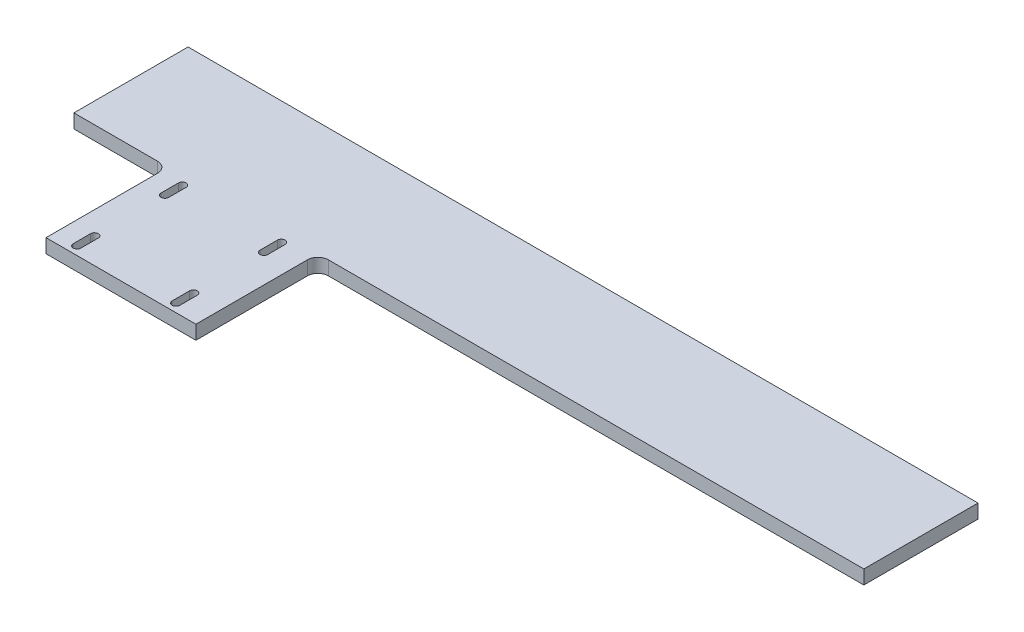
SolidWorks part; units mm, degrees
ref_plane "前视基准面" through (0, 0, 0) normal (0, 0, 1) x (1, 0, 0)
ref_plane "上视基准面" through (0, 0, 0) normal (0, 1, 0) x (1, 0, 0)
ref_plane "右视基准面" through (0, 0, 0) normal (1, 0, 0) x (0, 0, -1)
sketch "草图1" plane through (0, 0, 0) normal (0, 1, 0) x (1, 0, 0)
  line L1 (-1133, -163.75) -> (1133, -163.75)
  line L2 (-1133, -163.75) -> (-1133, 163.75)
  line L3 (-1133, 163.75) -> (1133, 163.75)
  line L4 (1133, -163.75) -> (1133, 163.75)
  line L5 (-1133, -163.75) -> (1133, 163.75) construction
  line L6 (-1133, 163.75) -> (1133, -163.75) construction
  point P0 (0, 0)
  dimension "D1" = 2266
  dimension "D2" = 327.5
extrude "凸台-拉伸1" add sketch "草图1" along normal blind 40
sketch "草图2" plane through (0, 40, 0) normal (0, 1, 0) x (1, 0, 0)
  line L0 (-1133, -163.75) -> (1133, -163.75) construction
  line L1 (-433, -163.75) -> (-863, -163.75)
  line L2 (-433, -163.75) -> (-433, -513.75)
  line L3 (-433, -513.75) -> (-863, -513.75)
  line L4 (-863, -163.75) -> (-863, -513.75)
  line L5 (-1133, 163.75) -> (-1133, -163.75) construction
  dimension "D1" = 700
  dimension "D2" = 430
  dimension "D3" = 350
extrude "凸台-拉伸2" add sketch "草图2" against normal blind 40
sketch "草图3" plane through (0, 40, 0) normal (0, 1, 0) x (1, 0, 0)
  line L0 (-514, -187.75) -> (-514, -237.75) construction
  line L1 (-503, -187.75) -> (-503, -237.75)
  line L2 (-525, -187.75) -> (-525, -237.75)
  line L3 (-433, -513.75) -> (-433, -163.75) construction
  line L4 (-514, -439.75) -> (-514, -489.75) construction
  line L7 (-863, -513.75) -> (-433, -513.75) construction
  line L8 (-798, -187.75) -> (-798, -237.75) construction
  line L9 (-787, -187.75) -> (-787, -237.75)
  line L10 (-809, -187.75) -> (-809, -237.75)
  line L11 (-798, -439.75) -> (-798, -489.75) construction
  line L12 (-787, -439.75) -> (-787, -489.75)
  line L13 (-809, -439.75) -> (-809, -489.75)
  line L14 (-503, -439.75) -> (-503, -489.75)
  line L15 (-525, -439.75) -> (-525, -489.75)
  line L16 (-1133, 163.75) -> (-1133, -163.75) construction
  line L17 (1133, 163.75) -> (-1133, 163.75) construction
  arc A0 (-503, -187.75) -> (-525, -187.75) centre (-514, -187.75) ccw
  arc A1 (-525, -237.75) -> (-503, -237.75) centre (-514, -237.75) ccw
  circle A2 centre (-514, -187.75) radius 11 construction
  arc A7 (-787, -187.75) -> (-809, -187.75) centre (-798, -187.75) ccw
  arc A8 (-809, -237.75) -> (-787, -237.75) centre (-798, -237.75) ccw
  circle A9 centre (-798, -187.75) radius 11 construction
  arc A10 (-787, -439.75) -> (-809, -439.75) centre (-798, -439.75) ccw
  arc A11 (-809, -489.75) -> (-787, -489.75) centre (-798, -489.75) ccw
  circle A12 centre (-798, -439.75) radius 11 construction
  arc A13 (-503, -439.75) -> (-525, -439.75) centre (-514, -439.75) ccw
  arc A14 (-525, -489.75) -> (-503, -489.75) centre (-514, -489.75) ccw
  circle A15 centre (-514, -439.75) radius 11 construction
  point P2 (-514, -212.75)
  point P12 (-514, -464.75)
  point P23 (-798, -212.75)
  point P32 (-798, -464.75)
  dimension "D6" = 11
  dimension "D8" = 25
  dimension "D9" = 11
  dimension "D11" = 25
  dimension "D4" = 11
  dimension "D12" = 25
  dimension "D1" = 22
  dimension "D2" = 50
  dimension "D3" = 25
  dimension "D5" = 50
  dimension "D7" = 50
  dimension "D10" = 50
  dimension "D13" = 81
  dimension "D14" = 49
  dimension "D15" = 252
  dimension "D16" = 252
extrude "切除-拉伸1" cut sketch "草图3" against normal through all
fillet "圆角1" radius 30 2 edges at (-863, 20, 163.75) (-433, 20, 163.75)
